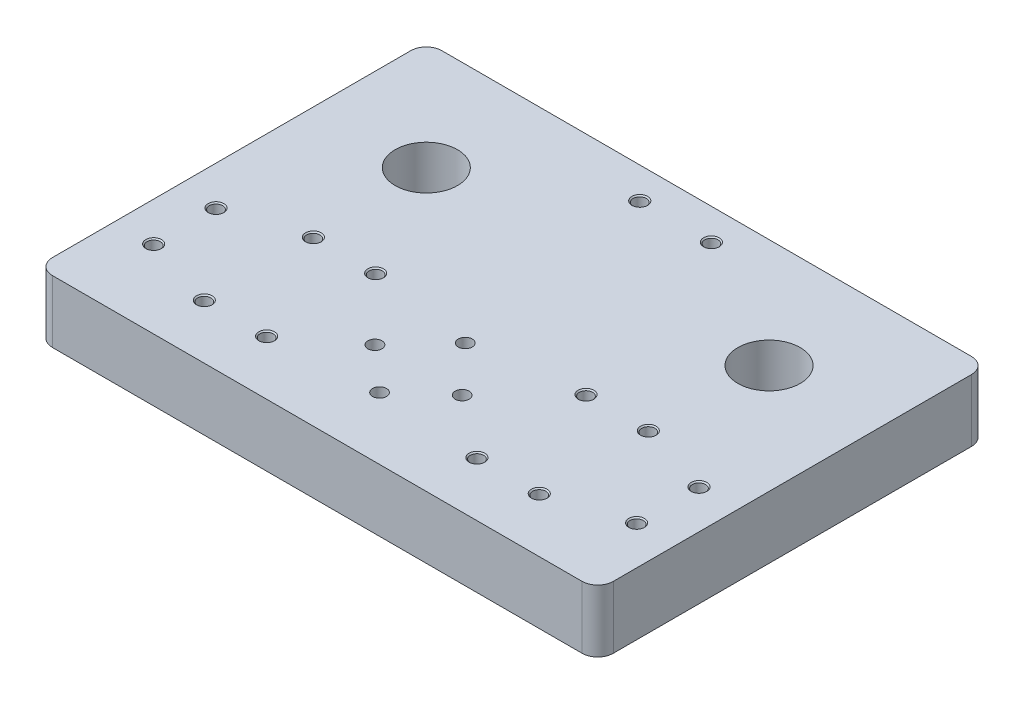
from build123d import *

# Parameters (mm, degrees)
SKETCH1_R                    = 20
SKETCH1_R_2                  = 4.5
BOSS_EXTRUDE1_DEPTH          = 40
SKETCH2_R                    = 7
CUT_EXTRUDE1_DEPTH           = 9
M10_TAPPED_HOLE1_D           = 8.5
M10_TAPPED_HOLE1_DEPTH       = 27.5
M10_TAPPED_HOLE1_CSINK_D     = 10.05
M10_TAPPED_HOLE1_CSINK_ANGLE = 90
M10_TAPPED_HOLE1_TIP         = 2.553657631


with BuildPart() as part:
    # Sketch1 → Boss-Extrude1 (new body)
    with BuildSketch(Plane(origin=(0, 0, 0), x_dir=(1, 0, 0), z_dir=(0, 1, 0))):
        with BuildLine():
            Line((-170, -125), (170, -125))
            ThreePointArc((170, -125), (177.071067812, -122.071067812), (180, -115))
            Line((180, -115), (180, 115))
            ThreePointArc((180, 115), (177.071067812, 122.071067812), (170, 125))
            Line((170, 125), (-170, 125))
            ThreePointArc((-170, 125), (-177.071067812, 122.071067812), (-180, 115))
            Line((-180, 115), (-180, -115))
            ThreePointArc((-180, -115), (-177.071067812, -122.071067812), (-170, -125))
        make_face()
        with Locations(Location((-110, 55, 0), (0, 0, 270))):
            Circle(SKETCH1_R, mode=Mode.SUBTRACT)
        with Locations(Location((110, 55, 0), (0, 0, 270))):
            Circle(SKETCH1_R, mode=Mode.SUBTRACT)
        with Locations(Location((0, -85, 0), (0, 0, 270))):
            Circle(SKETCH1_R_2, mode=Mode.SUBTRACT)
        with Locations(Location((0, -30, 0), (0, 0, 270))):
            Circle(SKETCH1_R_2, mode=Mode.SUBTRACT)
        with Locations(Location((28, -60, 0), (0, 0, 270))):
            Circle(SKETCH1_R_2, mode=Mode.SUBTRACT)
        with Locations(Location((-28, -60, 0), (0, 0, 270))):
            Circle(SKETCH1_R_2, mode=Mode.SUBTRACT)
    extrude(amount=BOSS_EXTRUDE1_DEPTH)

    # Sketch2 → Cut-Extrude1 (cut)
    with BuildSketch(Plane.XZ):
        with Locations(Location((0, 30, 0), (0, 0, 270))):
            Circle(SKETCH2_R)
        with Locations(Location((-28, 60, 0), (0, 0, 270))):
            Circle(SKETCH2_R)
        with Locations(Location((0, 85, 0), (0, 0, 270))):
            Circle(SKETCH2_R)
        with Locations(Location((28, 60, 0), (0, 0, 270))):
            Circle(SKETCH2_R)
    extrude(amount=-CUT_EXTRUDE1_DEPTH, mode=Mode.SUBTRACT)

    # M10 Tapped Hole1
    with Locations(Plane(origin=(0, 40, 0), x_dir=(1, 0, 0), z_dir=(0, 1, 0))):
        with Locations((-23, 105), (-155, -35), (-155, -75), (-107.5, -20), (-67.5, -20), (-107.5, -90), (-67.5, -90), (155, -75), (155, -35), (67.5, -90), (107.5, -90), (67.5, -20), (107.5, -20), (23, 105)):
            CounterSinkHole(M10_TAPPED_HOLE1_D / 2, M10_TAPPED_HOLE1_CSINK_D / 2, depth=M10_TAPPED_HOLE1_DEPTH, counter_sink_angle=M10_TAPPED_HOLE1_CSINK_ANGLE)
            with Locations((0, 0, -(M10_TAPPED_HOLE1_DEPTH + M10_TAPPED_HOLE1_TIP / 2))):  # 118° drill point
                Cone(0, M10_TAPPED_HOLE1_D / 2, M10_TAPPED_HOLE1_TIP, mode=Mode.SUBTRACT)


solid = part.part
